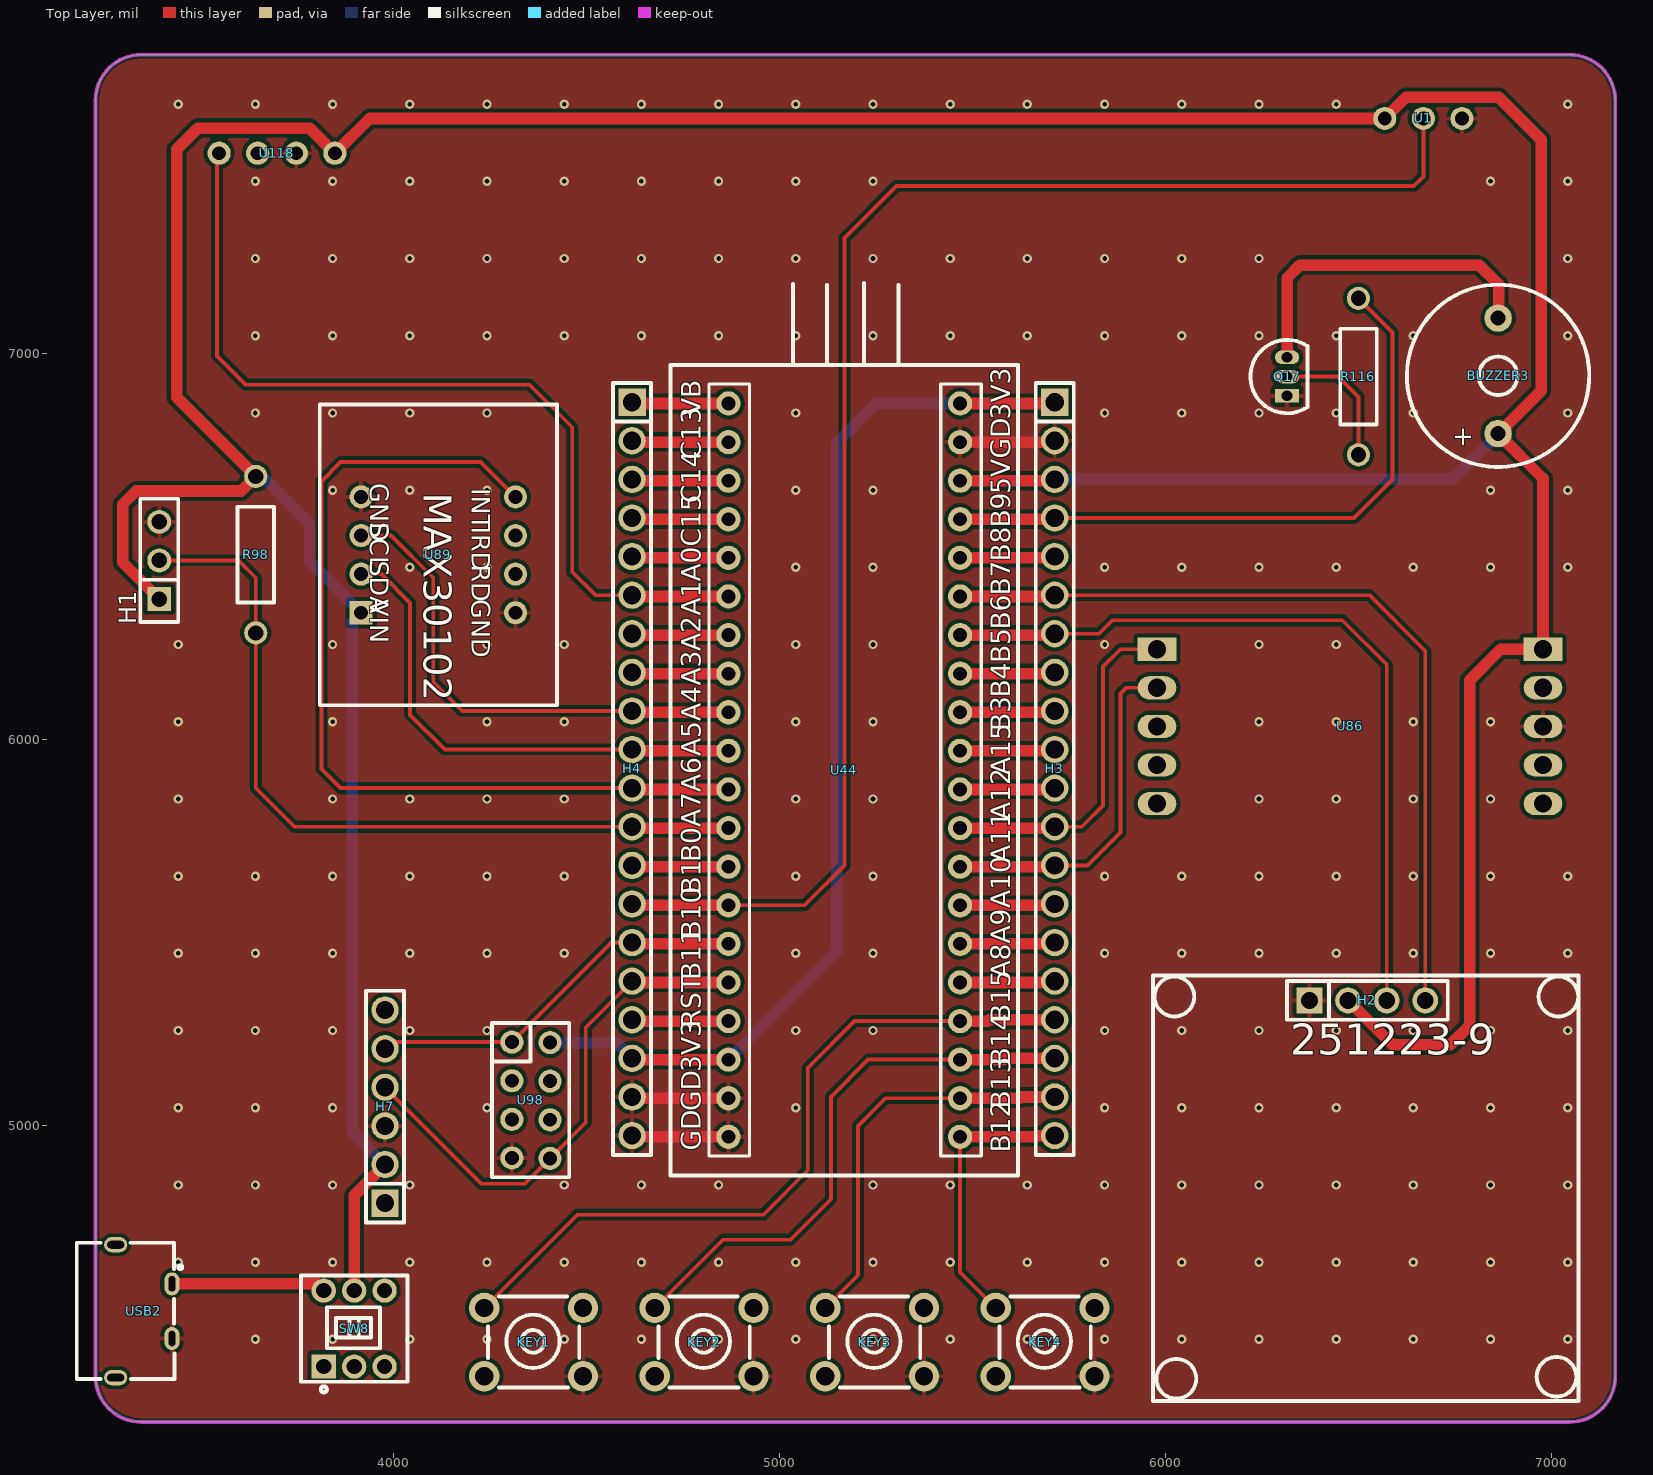
[diagram p0: Top Layer view]
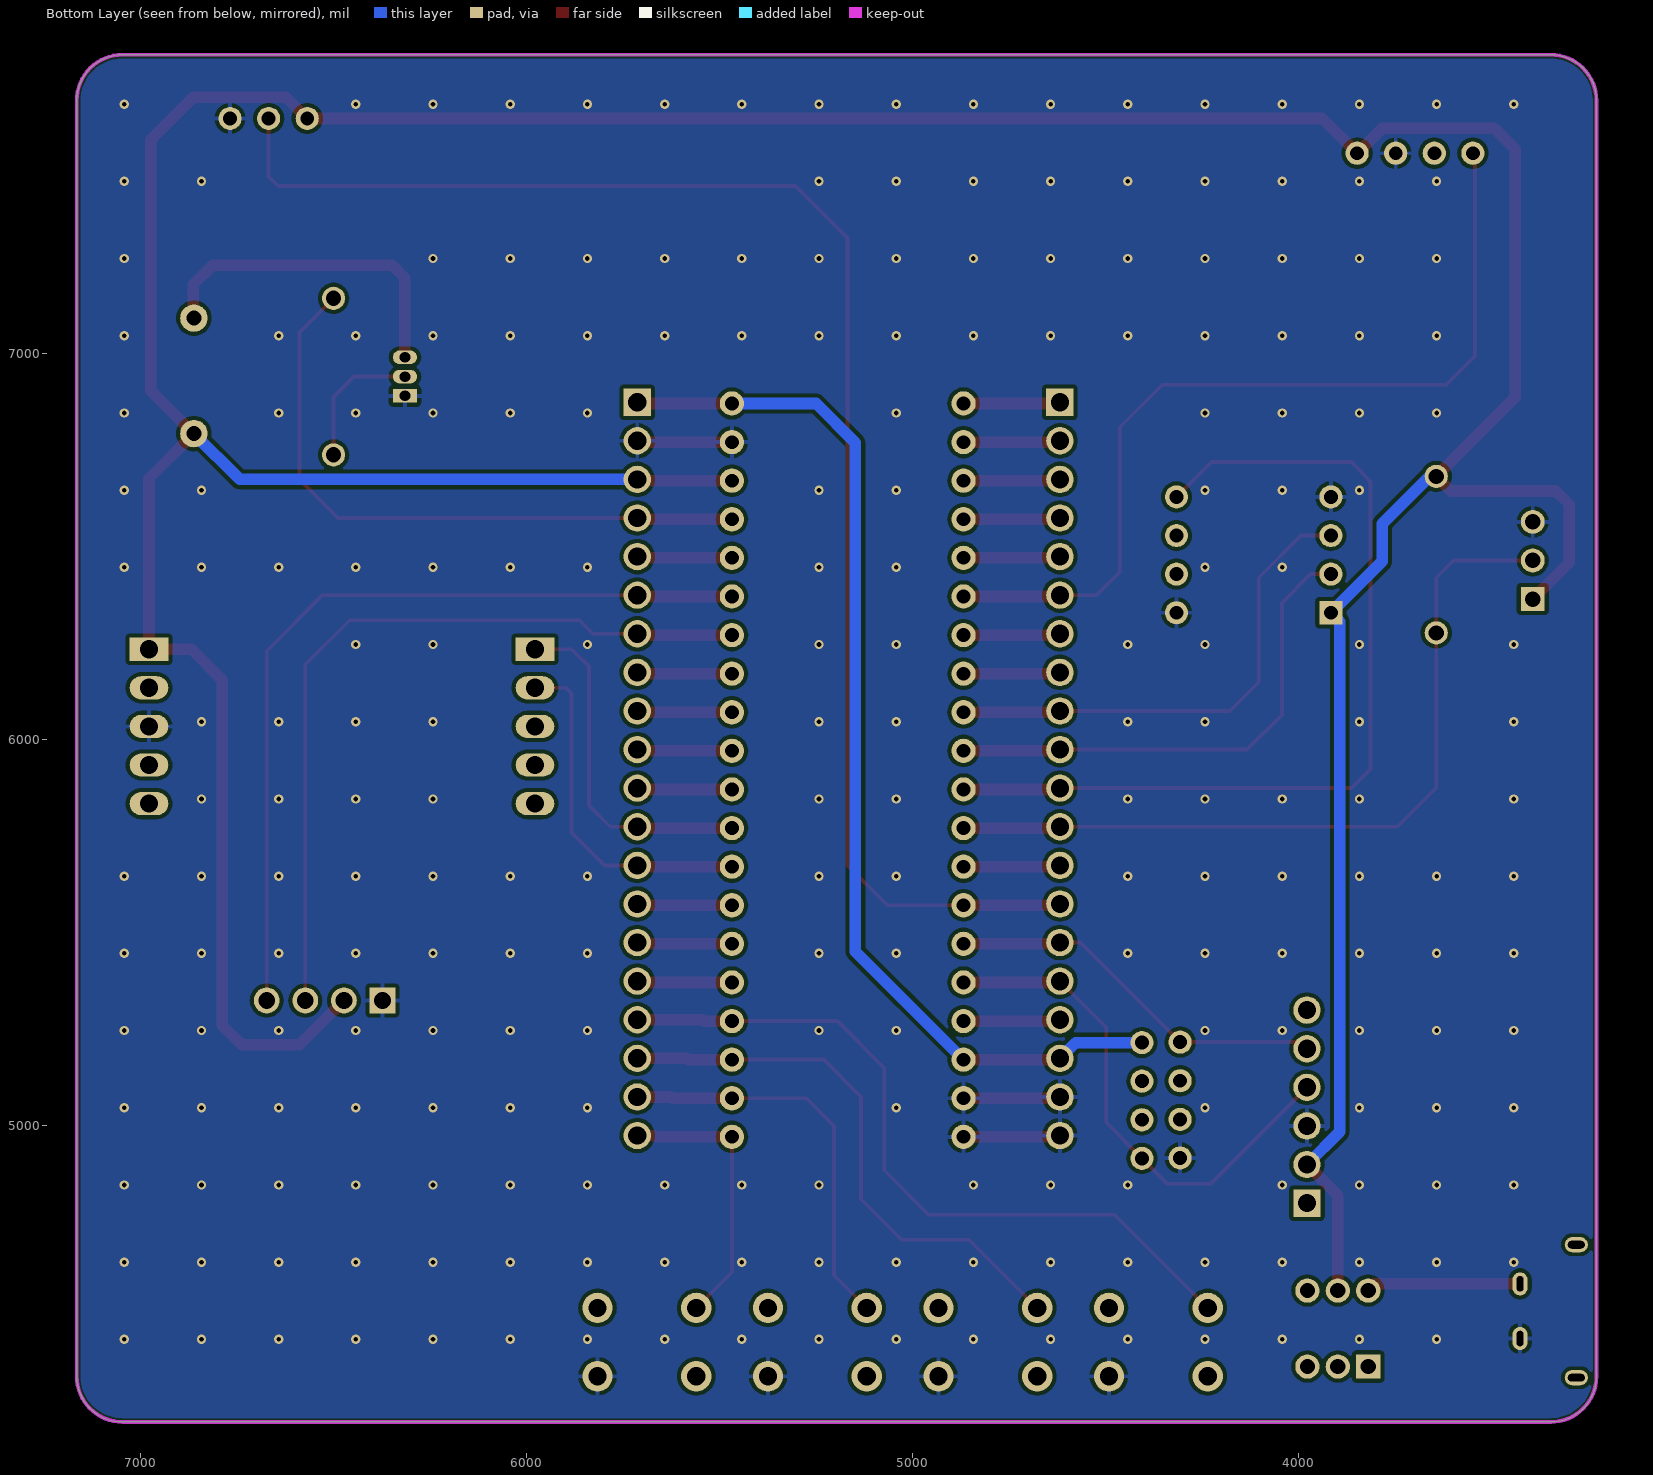
[diagram p1: Bottom Layer view, seen from below]
# Altium PCB MISC51907.pcbdoc
Units mil, origin at the board's own origin, x right, y up, seen from the top; angles counter-clockwise.
Board outline 3937.01 x 3542.01 mil, 2 copper layers (Top Layer, Bottom Layer), stack 62.206 mil thick; 21 components, 40 nets, 161 pads, 229 vias.

## Layer stack, top to bottom
Top Solder Mask Layer: solder mask 0.394, Dk 3.3
Top Layer: signal copper 1.379
Dielectric1: surface 59.449, FR4, Dk 4.5
Bottom Layer: signal copper 1.378
Bottom Solder Mask Layer: solder mask 0.394, Dk 3.3

## Board outline
3345.61,7775 ccw(c3345.61,7656.89) 3227.5,7656.89 3227.5,4351.1 ccw(c3345.61,4351.1) 3345.61,4232.99 7046.4,4232.99 ccw(c7046.4,4351.1) 7164.51,4351.1 7164.51,7656.89 ccw(c7046.4,7656.89) 7046.4,7775

## Design rules (kind name [scope] priority, off if disabled: settings)
BoardOutlineClearance copperThickness2oz_1 [All] p2 off: genericclearance=7.99 ignorepadtopadclearanceinfootprint=FALSE except(0: Arc-SplitContinuation Track-SplitContinuation SMDPad-SplitContinuation THPad-SplitContinuation Via-SplitContinuation Fill-SplitContinuation Region-SplitContinuation Poly-SplitContinuation Text-SplitContinuation Hole-SplitContinuation; 5.98: Arc-CutoutEdge Track-CutoutEdge SMDPad-CutoutEdge THPad-CutoutEdge Via-CutoutEdge Text-CutoutEdge; 6.9: Hole-OutlineEdge Hole-CutoutEdge; 10: Poly-OutlineEdge Poly-CutoutEdge; 11.81: Arc-OutlineEdge Track-OutlineEdge SMDPad-OutlineEdge THPad-OutlineEdge Via-OutlineEdge Fill-OutlineEdge Region-OutlineEdge Text-OutlineEdge Fill-CutoutEdge Region-CutoutEdge)
BoardOutlineClearance Plane_innerPlane_1 [All] p4 off: genericclearance=4.02 ignorepadtopadclearanceinfootprint=FALSE except(0: Arc-SplitContinuation Track-SplitContinuation SMDPad-SplitContinuation THPad-SplitContinuation Via-SplitContinuation Fill-SplitContinuation Region-SplitContinuation Poly-SplitContinuation Text-SplitContinuation Hole-SplitContinuation; 5.98: Arc-CutoutEdge Track-CutoutEdge SMDPad-CutoutEdge THPad-CutoutEdge Via-CutoutEdge Text-CutoutEdge; 6.9: Hole-OutlineEdge Hole-CutoutEdge; 10: Poly-OutlineEdge Poly-CutoutEdge; 11.81: Arc-OutlineEdge Track-OutlineEdge SMDPad-OutlineEdge THPad-OutlineEdge Via-OutlineEdge Fill-OutlineEdge Region-OutlineEdge Text-OutlineEdge Fill-CutoutEdge Region-CutoutEdge)
BoardOutlineClearance Copper_copperRegion_1 [All] p6 off: genericclearance=4.02 ignorepadtopadclearanceinfootprint=FALSE except(0: Arc-SplitContinuation Track-SplitContinuation SMDPad-SplitContinuation THPad-SplitContinuation Via-SplitContinuation Fill-SplitContinuation Region-SplitContinuation Poly-SplitContinuation Text-SplitContinuation Hole-SplitContinuation; 5.98: Arc-CutoutEdge Track-CutoutEdge SMDPad-CutoutEdge THPad-CutoutEdge Via-CutoutEdge Text-CutoutEdge; 6.9: Hole-OutlineEdge Hole-CutoutEdge; 10: Poly-OutlineEdge Poly-CutoutEdge; 11.81: Arc-OutlineEdge Track-OutlineEdge SMDPad-OutlineEdge THPad-OutlineEdge Via-OutlineEdge Fill-OutlineEdge Region-OutlineEdge Text-OutlineEdge Fill-CutoutEdge Region-CutoutEdge)
BoardOutlineClearance copperThickness1oz_1 [All] p8: genericclearance=4.02 ignorepadtopadclearanceinfootprint=FALSE except(0: Arc-SplitContinuation Track-SplitContinuation SMDPad-SplitContinuation THPad-SplitContinuation Via-SplitContinuation Fill-SplitContinuation Region-SplitContinuation Poly-SplitContinuation Text-SplitContinuation Hole-SplitContinuation; 5.98: Arc-CutoutEdge Track-CutoutEdge SMDPad-CutoutEdge THPad-CutoutEdge Via-CutoutEdge Text-CutoutEdge; 6.9: Hole-OutlineEdge Hole-CutoutEdge; 10: Poly-OutlineEdge Poly-CutoutEdge; 11.81: Arc-OutlineEdge Track-OutlineEdge SMDPad-OutlineEdge THPad-OutlineEdge Via-OutlineEdge Fill-OutlineEdge Region-OutlineEdge Text-OutlineEdge Fill-CutoutEdge Region-CutoutEdge)
Clearance copperThickness2oz [All] p1 off: gap=7.99 ignorepadtopadclearanceinfootprint=FALSE except(5.98: SMDPad-Track SMDPad-SMDPad THPad-Track SMDPad-THPad THPad-THPad Track-Via SMDPad-Via THPad-Via Via-Via Fill-SMDPad Region-SMDPad Fill-THPad Region-THPad Fill-Via Region-Via Fill-Fill Fill-Region Region-Region Arc-Track Arc-SMDPad Arc-THPad Arc-Via Fill-Arc Region-Arc Arc-Arc Text-Track SMDPad-Text Text-THPad Text-Via Fill-Text Region-Text Arc-Text Text-Text; 6.9: Hole-Track Hole-SMDPad Hole-THPad Hole-Via Fill-Hole Region-Hole Hole-Arc Hole-Text; 10: Poly-Track Poly-SMDPad Poly-THPad Poly-Via Poly-Fill Poly-Region Poly-Poly Poly-Arc Poly-Text Poly-Hole; 11.81: Fill-Track Region-Track)
Clearance Plane_innerPlane [All] p3 off: gap=4.02 ignorepadtopadclearanceinfootprint=FALSE except(5.98: SMDPad-Track SMDPad-SMDPad THPad-Track SMDPad-THPad THPad-THPad Track-Via SMDPad-Via THPad-Via Via-Via Fill-SMDPad Region-SMDPad Fill-THPad Region-THPad Fill-Via Region-Via Fill-Fill Fill-Region Region-Region Arc-Track Arc-SMDPad Arc-THPad Arc-Via Fill-Arc Region-Arc Arc-Arc Text-Track SMDPad-Text Text-THPad Text-Via Fill-Text Region-Text Arc-Text Text-Text; 6.9: Hole-Track Hole-SMDPad Hole-THPad Hole-Via Fill-Hole Region-Hole Hole-Arc Hole-Text; 10: Poly-Track Poly-SMDPad Poly-THPad Poly-Via Poly-Fill Poly-Region Poly-Poly Poly-Arc Poly-Text Poly-Hole; 11.81: Fill-Track Region-Track)
Clearance Copper_copperRegion [All] p5 off: gap=4.02 ignorepadtopadclearanceinfootprint=FALSE except(5.98: SMDPad-Track SMDPad-SMDPad THPad-Track SMDPad-THPad THPad-THPad Track-Via SMDPad-Via THPad-Via Via-Via Fill-SMDPad Region-SMDPad Fill-THPad Region-THPad Fill-Via Region-Via Fill-Fill Fill-Region Region-Region Arc-Track Arc-SMDPad Arc-THPad Arc-Via Fill-Arc Region-Arc Arc-Arc Text-Track SMDPad-Text Text-THPad Text-Via Fill-Text Region-Text Arc-Text Text-Text; 6.9: Hole-Track Hole-SMDPad Hole-THPad Hole-Via Fill-Hole Region-Hole Hole-Arc Hole-Text; 10: Poly-Track Poly-SMDPad Poly-THPad Poly-Via Poly-Fill Poly-Region Poly-Poly Poly-Arc Poly-Text Poly-Hole; 11.81: Fill-Track Region-Track)
Clearance copperThickness1oz [All] p7: gap=4.02 ignorepadtopadclearanceinfootprint=FALSE except(5.98: SMDPad-Track SMDPad-SMDPad THPad-Track SMDPad-THPad THPad-THPad Track-Via SMDPad-Via THPad-Via Via-Via Fill-SMDPad Region-SMDPad Fill-THPad Region-THPad Fill-Via Region-Via Fill-Fill Fill-Region Region-Region Arc-Track Arc-SMDPad Arc-THPad Arc-Via Fill-Arc Region-Arc Arc-Arc Text-Track SMDPad-Text Text-THPad Text-Via Fill-Text Region-Text Arc-Text Text-Text; 6.9: Hole-Track Hole-SMDPad Hole-THPad Hole-Via Fill-Hole Region-Hole Hole-Arc Hole-Text; 10: Poly-Track Poly-SMDPad Poly-THPad Poly-Via Poly-Fill Poly-Region Poly-Poly Poly-Arc Poly-Text Poly-Hole; 11.81: Fill-Track Region-Track)
DiffPairsRouting differentialPair [All] p1: maxlimit=6 minlimit=6 mostfreqgap=6 toplayer_minwidth=5 toplayer_prefwidth=10 toplayer_maxwidth=100 toplayer_mingap=6 toplayer_prefgap=6 toplayer_maxgap=6 bottomlayer_minwidth=5 bottomlayer_prefwidth=10 bottomlayer_maxwidth=100 bottomlayer_mingap=6 bottomlayer_prefgap=6 bottomlayer_maxgap=6 maxuncoupledlength=10
HoleToHoleClearance otherClearance [All] p1: gap=11.81 allowstackedmicrovias=TRUE
Length netLength [All] p1: minlimit=0 maxlimit=0
PasteMaskExpansion pasteMaskExpansion [All] p1: expansion=0
PlaneConnect innerPlane [All] p1: planeconnectstyle=Relief reliefexpansion=20 reliefentries=4 reliefconductorwidth=10 reliefairgap=10
PolygonConnect copperRegion [All] p1: connectstyle=Relief reliefconductorwidth=10 reliefentries=4 polygonreliefangle="90 Angle" airgapwidth=10 via.connectstyle=Relief via.reliefconductorwidth=10 via.reliefentries=4 via.polygonreliefangle="90 Angle" via.airgapwidth=10
RoutingVias viaSize [All] p1: holewidth=12.01 width=24.02 viastyle="Through Hole" minholewidth=11.81 minwidth=19.68 maxholewidth=248.03 maxwidth=393.7
SolderMaskExpansion solderMaskExpansion [IsVia] p1: expansion=-1000 istentingtop=TRUE
SolderMaskExpansion solderMaskExpansion [All] p2: expansion=2 istentingtop=FALSE
Width copperThickness2oz_2 [All] p1 off: maxlimit=100 minlimit=8 preferedwidth=10
Width copperThickness1oz_2 [All] p2: maxlimit=100 minlimit=5 preferedwidth=10

## Components (designator, comment, footprint, x,y, rotation, side; value= is the part's Value field where it differs from the comment)
BUZZER3 "2.3kHz" BUZ-TH_BD12.0-P7.60-D0.6-FD 6861.18,6943.16 r90 top
H1 "" HDR-TH_3P-P2.54-V-F 3392.5,6465 r90 top
H2 "2.54-1*4P female" HDR-TH_4P-P2.54-V-F 6522.5,5325 r0 top
H3 "" HDR-TH_20P-P2.54-V-M-1 5712.5,5925 r270 top
H4 "" HDR-TH_20P-P2.54-V-M-1 4617.5,5925 r270 top
H7 "" HDR-TH_6P-P2.54-V-M-1 3977.5,5050 r90 top
KEY1 "Button 1" KEY-TH_4P-L6.0-W6.0-P4.50-LS7.5 4362.5,4440 r0 top
KEY2 "Button 5" KEY-TH_4P-L6.0-W6.0-P4.50-LS7.5 4804.17,4440 r0 top
KEY3 "Button 2" KEY-TH_4P-L6.0-W6.0-P4.50-LS7.5 5245.83,4440 r0 top
KEY4 "Button 4" KEY-TH_4P-L6.0-W6.0-P4.50-LS7.5 5687.5,4440 r0 top
Q17 "" S8050_TO_92 6314.33,6941.32 r90 top
R98 "4.7kΩ" Res_1/4W 3642.5,6480 r90 top
R116 "1kΩ" Res_1/4W 6499.33,6941.32 r270 top
SW8 "TK-6700-1" SW-TH_TK-6700-1 3897.5,4475 r0 top
U1 "" 温湿度 6667.5,7610 r180 top
U44 "" STM32最小系统板 5207.1,6178.15 r0 top
U86 "" ADXL345 6472.5,6060 r0 top
U89 "" MAX30102 4062.5,6530 r270 top
U98 "" WiFi封装 4097.5,5065 r90 top
U118 "" MQ-X插件 3697.5,7520 r90 top
USB2 "KH-TYPE-C-2P" USB-SMD_KH-TYPE-C-2P 3352.5,4520 r270 top

## Footprints (in the part's own frame and the unit in brackets; to place one, negate y for a bottom-side part, rotate by r counter-clockwise, add the part's x,y. Pads: shape width x height; smd on the part's side, far side on the other; paste and mask are expansions set on the pad)
ADXL345 [mil]
  rect 100x60 hole 47.24: 1(-495,175) 10(505,175)
  oval 100x60 hole 47.24: 2(-495,75) 3(-495,-25) 4(-495,-125) 5(-495,-225) 6(505,-225) 7(505,-125) 8(505,-25) 9(505,75)
BUZ-TH_BD12.0-P7.60-D0.6-FD [mm]
  round 1.8 hole 1 paste+0 mask+0.051: 1(-3.8,0) 2(3.8,0)
  silkscreen extent -6,-6 6,6
HDR-TH_3P-P2.54-V-F [mil]
  rect 62x62 hole 40.16: 1(-100,0)
  round 62 hole 40.16: 2(0,0) 3(100,0)
  silkscreen extent -160,-49 160,49
HDR-TH_4P-P2.54-V-F [mm]
  rect 1.7x1.7 hole 1.1: 1(-3.81,0)
  round 1.7 hole 1.1: 2(-1.27,0) 3(1.27,0) 4(3.81,0)
  silkscreen extent -14.1,-26.35 13.9,1.65
HDR-TH_6P-P2.54-V-M-1 [mm]
  rect 1.8x1.8 hole 1.2: 1(-6.35,0)
  round 1.8 hole 1.2: 2(-3.81,0) 3(-1.27,0) 4(1.27,0) 5(3.81,0) 6(6.35,0)
  silkscreen extent -7.62,-1.25 7.62,1.25
HDR-TH_20P-P2.54-V-M-1 [mm]
  rect 1.8x1.8 hole 1.2: 1(-24.13,0)
  round 1.8 hole 1.2: 2(-21.59,0) 3(-19.05,0) 4(-16.51,0) 5(-13.97,0) 6(-11.43,0) 7(-8.89,0) 8(-6.35,0) 9(-3.81,0) 10(-1.27,0) 11(1.27,0) 12(3.81,0) 13(6.35,0) 14(8.89,0) 15(11.43,0) 16(13.97,0) 17(16.51,0) 18(19.05,0) 19(21.59,0) 20(24.13,0)
  silkscreen extent -25.4,-1.25 25.4,1.25
KEY-TH_4P-L6.0-W6.0-P4.50-LS7.5 [mm]
  round 2 hole 1.2 paste+0 mask+0.051: 1(-3.25,-2.25) 2(3.25,-2.25) 3(3.25,2.25) 4(-3.25,2.25)
  silkscreen extent -3,-3 3,3
MAX30102 [mil]
  round 60 hole 36 paste+0 mask+0: 1(200.48,252.99) 2(100.48,252.99) 3(0.48,252.99) 4(-99.52,252.99) 5(-99.52,-147.01) 6(0.48,-147.01) 7(100.48,-147.01)
  rect 60x60 hole 36 paste+0 mask+0: 8(200.47,-147.01)
  silkscreen extent -339,-254 440,360
MQ-X插件 [mil]
  round 60 hole 36: 1(0,150) 2(0,50) 3(0,-50) 4(0,-150)
Res_1/4W [mil]
  round 60 hole 39.37 paste+0 mask+2: 1(-202.76,0) 2(202.76,0)
  silkscreen extent -124,-47 124,47
S8050_TO_92 [mil]
  rect 35.4x63 hole 27.6 paste+0 mask+2: 1(-50,0)
  oval 35.4x63 hole 27.6 paste+0 mask+2: 2(0,0) 3(50,0)
  silkscreen extent -95,-53 95,95
STM32最小系统板 [mm]
  round 1.6 hole 0.9: 1(-8.634,17.614) 2(-8.634,15.074) 3(-8.634,12.534) 4(-8.634,9.994) 5(-8.634,7.454) 6(-8.634,4.914) 7(-8.634,2.374) 8(-8.634,-0.166) 9(-8.634,-2.706) 10(-8.634,-5.246) 11(-8.634,-7.786) 12(-8.634,-10.326) 13(-8.634,-12.866) 14(-8.634,-15.406) 15(-8.634,-17.946) 16(-8.634,-20.486) 17(-8.634,-23.026) 18(-8.634,-25.566) 19(-8.634,-28.106) 20(-8.634,-30.646) 21(6.606,17.614) 22(6.606,15.074) 23(6.606,12.534) 24(6.606,9.994) 25(6.606,7.454) 26(6.606,4.914) 27(6.606,2.374) 28(6.606,-0.166) 29(6.606,-2.706) 30(6.606,-5.246) 31(6.606,-7.786) 32(6.606,-10.326) 33(6.606,-12.866) 34(6.606,-15.406) 35(6.606,-17.946) 36(6.606,-20.486) 37(6.606,-23.026) 38(6.606,-25.566) 39(6.606,-28.106) 40(6.606,-30.646)
  silkscreen extent -12.44,-33.19 10.42,25.54
SW-TH_TK-6700-1 [mm]
  rect 1.6x1.6 hole 1 paste+0 mask+0.051: 1(-2,-2.5)
  round 1.6 hole 1 paste+0 mask+0.051: 2(0,-2.5) 3(2,-2.5)
  round 1.6 hole 1 copper offset 0,0 paste+0 mask+0.051: 4(-2,2.5) 5(0,2.5) 6(2,2.5)
  silkscreen extent -3.5,-4.2 3.5,3.5
USB-SMD_KH-TYPE-C-2P [mm]
  oval 1.524x1 hole 0.45 slot 1 at 0 deg paste+0 mask+0.05: 1(-1.8,1.85) 2(1.8,1.85)
  oval 1x1.524 hole 0.5 slot 1.1 at 90 deg paste+0 mask+0.05: 3(4.375,-1.85) 4(-4.375,-1.85)
  silkscreen extent -4.5,-4.41 4.46,2.53
WiFi封装 [mil]
  round 60 hole 36: 1(152.01,-208.54) 2(150.91,-307.4) 3(52.01,-208.54) 4(50.91,-307.4) 5(-47.99,-208.54) 6(-49.09,-307.4) 7(-147.99,-208.54) 8(-149.09,-307.4)
  silkscreen extent -198,-357 202,-157
温湿度 [mil]
  round 60 hole 36: 1(-100,0) 2(0,0) 3(100,0)

## Via types
v1: diameter 24.02, hole 12, Top Layer to Bottom Layer, 229 vias

## Nets (pads, with @x,y where several pads share a name; then routed paths per layer and width w, separated by ;. In a path a pad name is that pad's centre, name@x,y a point inside that pad or via, vN(x,y) a via of type N, cw(c..) or ccw(c..) an arc to the next point about the centre after c; other vN are vias at no path point)
3V3: H3.1 H4.18 U44.18 U44.21 U98.2 | length 2807.2
  Top Layer w30: H4.18@4612.5,5171.61 U44.18 ; U44.21 5709.11,6871.61 H3.1
  Bottom Layer w30: U98.2 4576.59,5215.91 H4.18 ; U44.18 5147.5,5451.93 5147.5,6770 5249.11,6871.61 U44.21
$1N362: H3.5 U44.25 | length 246.7
  Top Layer w30: U44.25 5709.11,6471.61 H3.5
$1N367: H3.8 U44.28 | length 246.7
  Top Layer w30: U44.28 5709.11,6171.61 H3.8
$1N368: H3.9 U44.29 | length 246.7
  Top Layer w30: U44.29 5709.11,6071.61 H3.9
$1N369: H3.10 U44.30 | length 246.7
  Top Layer w30: U44.30 5709.11,5971.61 H3.10
$1N370: H3.11 U44.31 | length 246.7
  Top Layer w30: U44.31 5709.11,5871.61 H3.11
$1N377: H3.16 U44.36 | length 246.7
  Top Layer w30: U44.36 5709.11,5371.61 H3.16
$1N386: H4.1 U44.1 | length 254.7
  Top Layer w30: H4.1@4612.5,6871.61 U44.1
$1N387: H4.2 U44.2 | length 254.7
  Top Layer w30: H4.2@4612.5,6771.61 U44.2
$1N388: H4.3 U44.3 | length 254.7
  Top Layer w30: H4.3@4612.5,6671.61 U44.3
$1N389: H4.4 U44.4 | length 254.7
  Top Layer w30: H4.4@4612.5,6571.61 U44.4
$1N406: H4.17 U44.17 | length 254.7
  Top Layer w30: H4.17@4612.5,5271.61 U44.17
$1N3404: Q17.2 R116.2 | length 356.6
  Top Layer w10: Q17.2 6446.18,6941.32 6499.33,6888.17 R116.2
$1N3407: BUZZER3.2 Q17.3 | length 875.9
  Top Layer w30: Q17.3 6314.33,7196.83 6347.5,7230 6812.5,7230 6862.5,7180 6862.5,7094.08 BUZZER3.2
+5V: BUZZER3.1 H1.1 H2.2 H3.3 H7.2 R98.2 SW8.5 U1.3 U44.23 U86.10 U89.8 U118.4 | length 11952.7
  Top Layer w30: H1.1 3297.5,6460 3297.5,6610 3332.5,6645 3604.74,6645 R98.2 3437.5,6887.76 3437.5,7530 3492.5,7585 3782.5,7585 U118.4 3937.5,7610 U1.3 6622.5,7665 6862.5,7665 6972.5,7555 6972.5,6904.87 BUZZER3.1 6977.5,6677.23 U86.10 6867.5,6235 6787.5,6155 6787.5,5260 6737.5,5210 6587.5,5210 H2.2 ; SW8.5 3897.5,4820 3924.68,4847.18 cw(c3942.07,4835.43) 3930.32,4852.82 H7.2 ; U44.23 5709.11,6671.61 H3.3
  Bottom Layer w30: R98.2 3659.74,6682.76 3782.5,6560 3782.5,6462.52 U89.8 3892.5,6306.53 3892.5,4985 H7.2 ; H3.3 6742.63,6675 BUZZER3.1
GND: H1.3 H2.1 H3.2 H4.19 H4.20 H7.3 KEY1.2 KEY2.2 KEY3.2 KEY4.2 Q17.1 U1.1 U44.19 U44.20 U44.22 U86.8 U89.1 U89.5 U98.7 U118.3 USB2.2 | length 756.1
  Top Layer w30: H4.20@4612.5,4971.61 U44.20 ; H4.19@4612.5,5071.61 U44.19 ; U44.22 5709.11,6771.61 H3.2
  other v1: 3641.6,4447.09 3841.6,4447.09 4041.6,4447.09 4241.6,4447.09 4441.6,4447.09 4641.6,4447.09 4841.6,4447.09 5041.6,4447.09 5241.6,4447.09 5441.6,4447.09 5641.6,4447.09 5841.6,4447.09 6041.6,4447.09 6241.6,4447.09 6441.6,4447.09 6641.6,4447.09 6841.6,4447.09 7041.6,4447.09 3441.6,4647.09 3641.6,4647.09 3841.6,4647.09 4041.6,4647.09 4241.6,4647.09 4441.6,4647.09 4641.6,4647.09 4841.6,4647.09 5041.6,4647.09 5241.6,4647.09 5441.6,4647.09 5641.6,4647.09 5841.6,4647.09 6041.6,4647.09 6241.6,4647.09 6441.6,4647.09 6641.6,4647.09 6841.6,4647.09 7041.6,4647.09 3441.6,4847.09 3641.6,4847.09 3841.6,4847.09 4041.6,4847.09 4441.6,4847.09 4641.6,4847.09 4841.6,4847.09 5241.6,4847.09 5441.6,4847.09 5641.6,4847.09 5841.6,4847.09 6041.6,4847.09 6241.6,4847.09 6441.6,4847.09 6641.6,4847.09 6841.6,4847.09 7041.6,4847.09 3441.6,5047.09 3641.6,5047.09 3841.6,5047.09 4241.6,5047.09 5041.6,5047.09 5841.6,5047.09 6041.6,5047.09 6241.6,5047.09 6441.6,5047.09 6641.6,5047.09 6841.6,5047.09 7041.6,5047.09 3441.6,5247.09 3641.6,5247.09 3841.6,5247.09 4041.6,5247.09 4241.6,5247.09 5041.6,5247.09 5241.6,5247.09 5841.6,5247.09 6041.6,5247.09 6241.6,5247.09 6441.6,5247.09 6641.6,5247.09 6841.6,5247.09 7041.6,5247.09 3441.6,5447.09 3641.6,5447.09 3841.6,5447.09 4041.6,5447.09 4241.6,5447.09 4441.6,5447.09 5041.6,5447.09 5241.6,5447.09 5841.6,5447.09 6041.6,5447.09 6241.6,5447.09 6441.6,5447.09 6641.6,5447.09 6841.6,5447.09 7041.6,5447.09 3441.6,5647.09 3641.6,5647.09 3841.6,5647.09 4041.6,5647.09 4241.6,5647.09 4441.6,5647.09 5041.6,5647.09 5241.6,5647.09 5841.6,5647.09 6041.6,5647.09 6241.6,5647.09 6441.6,5647.09 6641.6,5647.09 6841.6,5647.09 7041.6,5647.09 3441.6,5847.09 3841.6,5847.09 4041.6,5847.09 4241.6,5847.09 4441.6,5847.09 5041.6,5847.09 5241.6,5847.09 6241.6,5847.09 6441.6,5847.09 6641.6,5847.09 6841.6,5847.09 3441.6,6047.09 3841.6,6047.09 4241.6,6047.09 4441.6,6047.09 5041.6,6047.09 5241.6,6047.09 6241.6,6047.09 6441.6,6047.09 6641.6,6047.09 6841.6,6047.09 3441.6,6247.09 3841.6,6247.09 4241.6,6247.09 4441.6,6247.09 5041.6,6247.09 5241.6,6247.09 5841.6,6247.09 6241.6,6247.09 6441.6,6247.09 4041.6,6447.09 4241.6,6447.09 5041.6,6447.09 5241.6,6447.09 5841.6,6447.09 6041.6,6447.09 6241.6,6447.09 6441.6,6447.09 6641.6,6447.09 6841.6,6447.09 7041.6,6447.09 3841.6,6647.09 4041.6,6647.09 4241.6,6647.09 5041.6,6647.09 5241.6,6647.09 6841.6,6647.09 7041.6,6647.09 3641.6,6847.09 3841.6,6847.09 4041.6,6847.09 4241.6,6847.09 5041.6,6847.09 5841.6,6847.09 6041.6,6847.09 6241.6,6847.09 6441.6,6847.09 6641.6,6847.09 7041.6,6847.09 3641.6,7047.09 3841.6,7047.09 4041.6,7047.09 4241.6,7047.09 4441.6,7047.09 4641.6,7047.09 4841.6,7047.09 5041.6,7047.09 5241.6,7047.09 5441.6,7047.09 5641.6,7047.09 5841.6,7047.09 6041.6,7047.09 6241.6,7047.09 6441.6,7047.09 6641.6,7047.09 7041.6,7047.09 3641.6,7247.09 3841.6,7247.09 4041.6,7247.09 4241.6,7247.09 4441.6,7247.09 4641.6,7247.09 4841.6,7247.09 5041.6,7247.09 5241.6,7247.09 5441.6,7247.09 5641.6,7247.09 5841.6,7247.09 6041.6,7247.09 6241.6,7247.09 7041.6,7247.09 3641.6,7447.09 3841.6,7447.09 4041.6,7447.09 4241.6,7447.09 4441.6,7447.09 4641.6,7447.09 4841.6,7447.09 5041.6,7447.09 5241.6,7447.09 6841.6,7447.09 7041.6,7447.09 3441.6,7647.09 3641.6,7647.09 3841.6,7647.09 4041.6,7647.09 4241.6,7647.09 4441.6,7647.09 4641.6,7647.09 4841.6,7647.09 5041.6,7647.09 5241.6,7647.09 5441.6,7647.09 5641.6,7647.09 5841.6,7647.09 6041.6,7647.09 6241.6,7647.09 6441.6,7647.09 7041.6,7647.09
PA0: H4.5 U44.5 | length 254.7
  Top Layer w30: H4.5@4612.5,6471.61 U44.5
PA1: H4.6 U44.6 U118.1 | length 2328.2
  Top Layer w10: U118.1 3542.5,7515 3542.5,6995 3617.5,6920 4352.5,6920 4462.5,6810 4462.5,6435 4522.5,6375 H4.6@4612.5,6375
  Top Layer w30: H4.6@4612.5,6371.61 U44.6
PA4: H4.9 U44.9 U89.6 | length 1298.1
  Top Layer w10: U89.6 3992.98,6529.52 4102.5,6420 4102.5,6150 4177.5,6075 H4.9@4612.5,6075
  Top Layer w30: H4.9@4612.5,6071.61 U44.9
PA5: H4.10 U44.10 U89.7 | length 1309.8
  Top Layer w10: U89.7 3967.98,6429.52 4042.5,6355 4042.5,6065 4132.5,5975 H4.10@4612.5,5975
  Top Layer w30: H4.10@4612.5,5971.61 U44.10
PA6: H4.11 U44.11 U89.4 | length 2381.6
  Top Layer w10: U89.4 4225.02,6720 3862.5,6720 3812.5,6670 3812.5,5925 3862.5,5875 H4.11@4612.5,5875
  Top Layer w30: H4.11@4612.5,5871.61 U44.11
PA7: H1.2 H4.12 R98.1 U44.12 | length 2079.7
  Top Layer w10: H1.2 3597.49,6465.01 3642.5,6420 R98.1 3642.5,5875 3742.5,5775 H4.12@4612.5,5775
  Top Layer w30: H4.12@4612.5,5771.61 U44.12
PA11: H3.13 U44.33 U86.2 | length 913.1
  Top Layer w10: H3.13 5797.5,5675 5882.5,5760 5882.5,6120 5897.5,6135 U86.2
  Top Layer w30: U44.33 5709.11,5671.61 H3.13
PA12: H3.12 U44.32 U86.1 | length 913.1
  Top Layer w10: H3.12 5782.5,5775 5837.5,5830 5837.5,6190 5882.5,6235 U86.1
  Top Layer w30: U44.32 5709.11,5771.61 H3.12
PB0: H4.13 U44.13 | length 254.7
  Top Layer w30: H4.13@4612.5,5671.61 U44.13
PB1: H4.14 U1.2 U44.14 | length 3939.1
  Top Layer w10: U44.14 5064.11,5571.61 5167.5,5675 5167.5,7300 5302.5,7435 6642.5,7435 6667.5,7460 U1.2
  Top Layer w30: H4.14@4612.5,5571.61 U44.14
PB6: H2.3 H3.7 U44.27 | length 2038.9
  Top Layer w10: H3.7 5827.5,6275 5862.5,6310 6457.5,6310 6572.5,6195 H2.3
  Top Layer w30: U44.27 5709.11,6271.61 H3.7
PB7: H2.4 H3.6 U44.26 | length 2171.8
  Top Layer w10: H3.6 6527.5,6375 6672.5,6230 H2.4
  Top Layer w30: U44.26 5709.11,6371.61 H3.6
PB9: H3.4 R116.1 U44.24 | length 1668.7
  Top Layer w10: H3.4 6487.5,6575 6587.5,6675 6587.5,7055.92 R116.1
  Top Layer w30: U44.24 5709.11,6571.61 H3.4
PB12: H3.20 KEY4.4 U44.40 | length 728
  Top Layer w10: U44.40 5467.18,4620.95 KEY4.4
  Top Layer w30: U44.40 5663.68,4971.61 5667.07,4975 H3.20
PB13: H3.19 KEY3.4 U44.39 | length 1047.5
  Top Layer w10: KEY3.4 5202.5,4613.2 5202.5,5000 5274.11,5071.61 U44.39
  Top Layer w30: U44.39 5622.26,5071.61 5625.65,5075 H3.19
PB14: H3.18 KEY2.4 U44.38 | length 1459.3
  Top Layer w10: KEY2.4 4852.64,4705 5027.5,4705 5132.5,4810 5132.5,5075 5229.11,5171.61 U44.38
  Top Layer w30: U44.38 5580.84,5171.61 5584.22,5175 H3.18
PB15: H3.17 KEY1.4 U44.37 | length 1942.4
  Top Layer w10: KEY1.4 4475.97,4770 4957.5,4770 5072.5,4885 5072.5,5150 5194.11,5271.61 U44.37
  Top Layer w30: U44.37 5539.42,5271.61 5542.8,5275 H3.17
U1_RX: H3.14 U44.34 | length 246.7
  Top Layer w30: U44.34 5709.11,5571.61 H3.14
U1_TX: H3.15 U44.35 | length 246.7
  Top Layer w30: U44.35 5709.11,5471.61 H3.15
U2_RX: H4.8 U44.8 | length 254.7
  Top Layer w30: H4.8@4612.5,6171.61 U44.8
U2_TX: H4.7 U44.7 | length 254.7
  Top Layer w30: H4.7@4612.5,6271.61 U44.7
U3_RX: H4.16 H7.4 U44.16 U98.8 | length 1354.2
  Top Layer w10: H7.4 4227.5,4850 4338.99,4850 U98.8 4497.5,5008.51 4497.5,5255 H4.16@4613.31,5370.81
  Top Layer w30: H4.16@4612.5,5371.61 U44.16
U3_TX: H4.15 H7.5 U44.15 U98.1 | length 1003.6
  Top Layer w10: H7.5 3994.51,5217.01 U98.1 4564.03,5475 H4.15@4612.5,5475
  Top Layer w30: H4.15@4612.5,5471.61 U44.15
VUSB: SW8.4 USB2.1 | length 400.7
  Top Layer w30: USB2.1 3801.32,4590.87 SW8.4
pads on no net: H7.1 H7.6 KEY1.1 KEY1.3 KEY2.1 KEY2.3 KEY3.1 KEY3.3 KEY4.1 KEY4.3 SW8.1 SW8.2 SW8.3 SW8.6 U86.3 U86.4 U86.5 U86.6 U86.7 U86.9 U89.2 U89.3 U98.3 U98.4 U98.5 U98.6 U118.2 USB2.3 USB2.4

## Polygon pours and split planes (outlines as drawn)
GND on Bottom Layer (solid, remove dead copper, pour order 2): 3137.5,7880 3137.5,3925 7282.5,3925 7282.5,7880
GND on Top Layer (solid, remove dead copper, pour order 0): 3000,3000 7482.5,3000 7482.5,8237.5 3000,8237.5

## Keep-outs
Board Outline Layer:
  the board outline again, w10

## Silkscreen, mask and mechanical layers (free items; w line width, h text height)
Top Silkscreen Layer:
  text "251223-9" at 6322.5,5185 h80